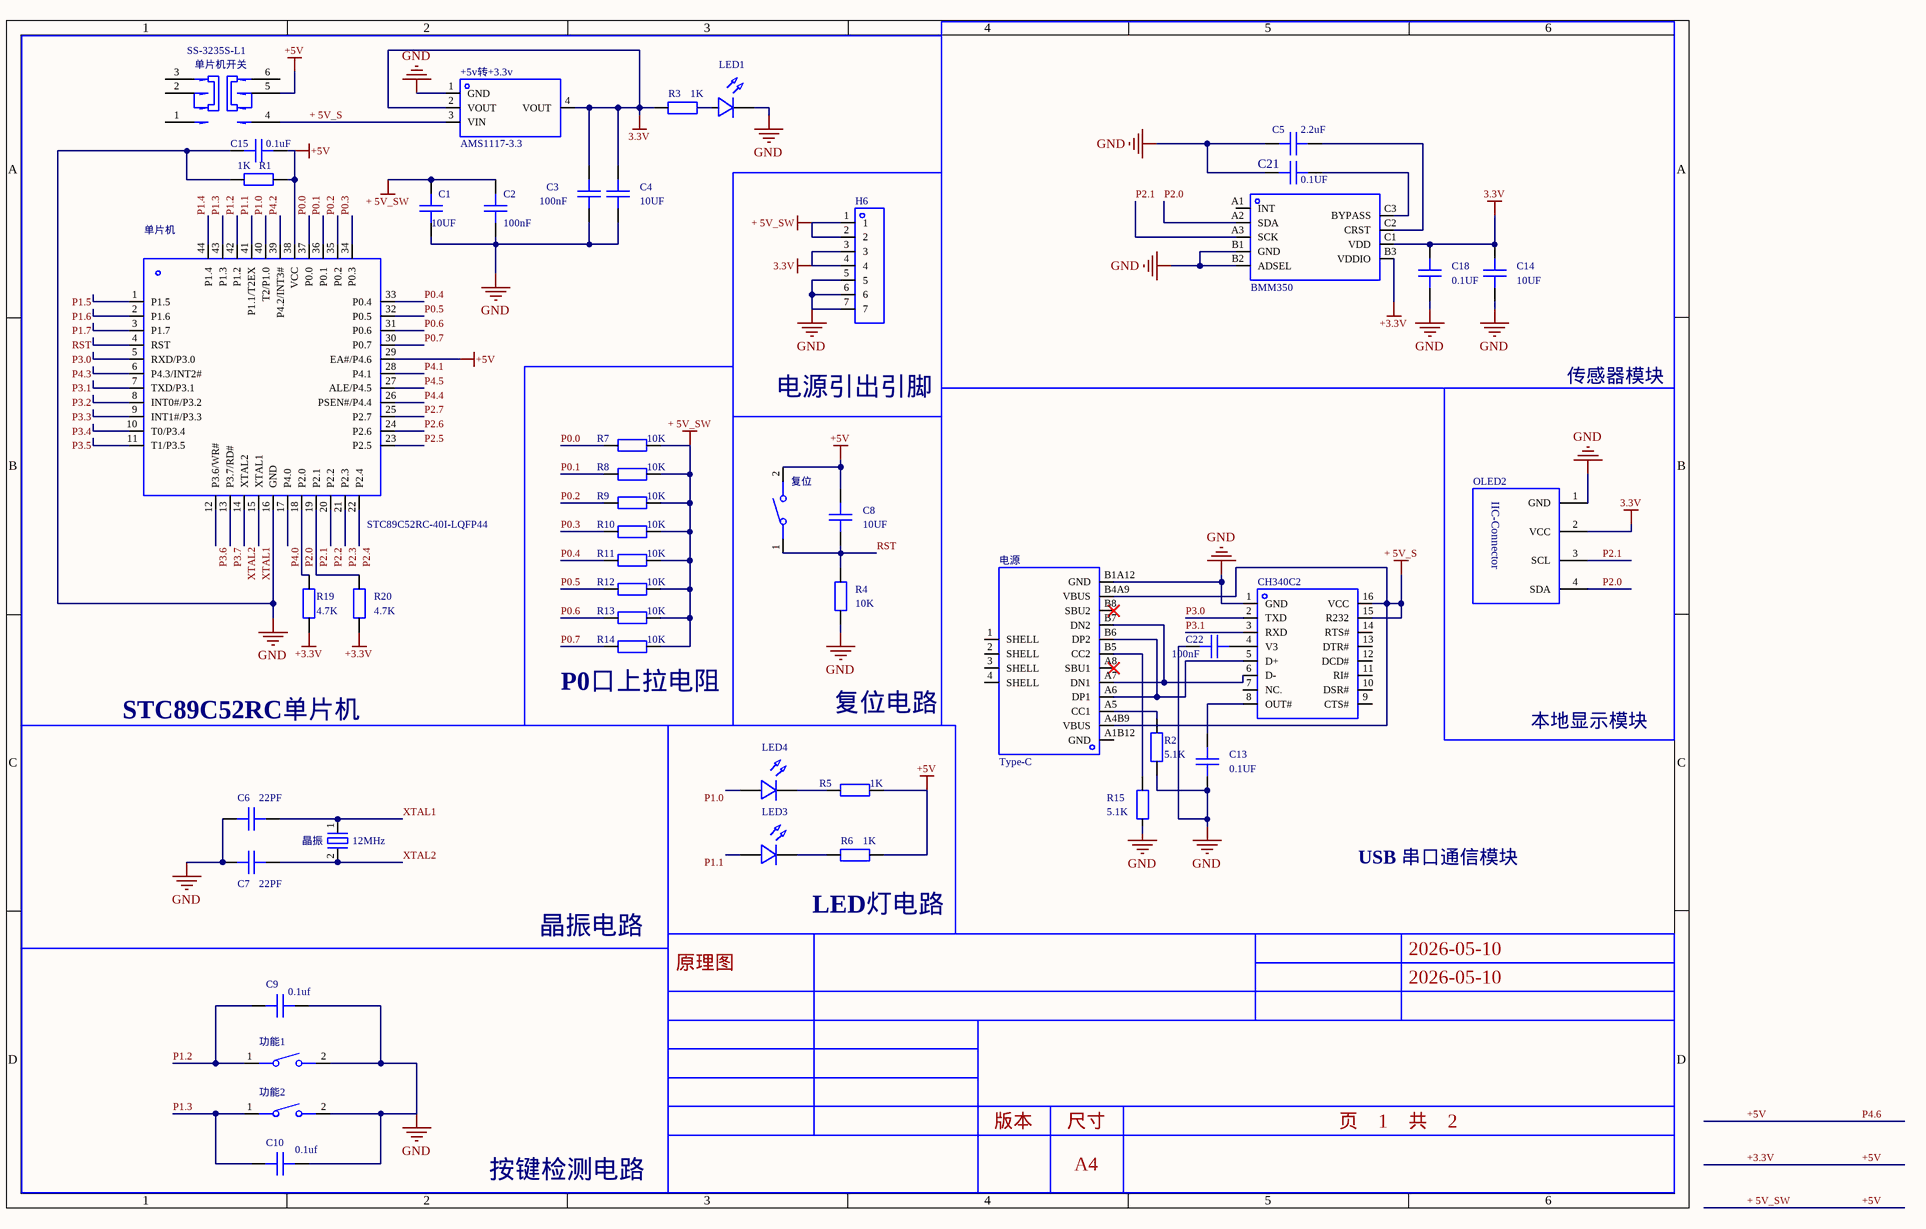
[diagram p0: MISC51448-3.schdoc]
# Altium project MISC51448-2.PrjPcb
1 sheet, 48 parts. Net scope: global (net labels, ports and power ports of the same name join across sheets).
Board file: MISC51448.pcbdoc

## Sheet MISC51448-3.schdoc
size 297 x 209 mm; Version: V1.0; @Project Name: MISC51448; @Page Count: 2; @Update Date: 2026-05-18; @Create Date: 2026-05-18; @Schematic Name: MISC51448; @Page No: 1; @Board Name: MISC51448; @Create Time: 00:24:12; @Update Time: 02:37:15; Size: A4

### Parts
+5v转+3.3v  AMS1117-3.3  [SOT-223-3_L6.5-W3.4-P2.30-LS7.0-BR]
C1  10UF  [C0805]
C2  100nF  [C0805]
C3  100nF  [C0805]
C4  10UF  [C0805]
C5  2.2uF  [C0805]
C6  22PF  [C0805]
C7  22PF  [C0805]
C8  10UF  [C0805]
C9  0.1uf  [C0805]
C10  0.1uf  [C0805]
C13  0.1UF  [C0805]
C14  10UF  [C0805]
C15  0.1uF  [C0805]
C18  0.1UF  [C0805]
C21  0.1UF  [C0805]
C22  100nF  [C0603]
CH340C2  CH340C  [SOP-16_L10.0-W3.9-P1.27-LS6.0-BL]  (value not drawn)
H6  (no value)  [HDR-TH_7P-P2.54-V-M]
LED1  (no value)  [LED_0805]
LED3  (no value)  [LED_0805]
LED4  (no value)  [LED_0805]
OLED2  0.96OLED_4P_MODULE_JX  [0.96OLED_4P]  (value not drawn)
R1  1K  [R0805]
R2  5.1K  [R0603]
R3  1K  [R0805]
R4  10K  [R0805]
R5  1K  [R0805]
R6  1K  [R0805]
R7  10K  [R0805]
R8  10K  [R0805]
R9  10K  [R0805]
R10  10K  [R0805]
R11  10K  [R0805]
R12  10K  [R0805]
R13  10K  [R0805]
R14  10K  [R0805]
R15  5.1K  [R0603]
R19  4.7K  [R0603]
R20  4.7K  [R0603]
U1  BMM350  [WLCSP-9_L1.3-W1.3-R3-C3-P0.40-TL]
功能1  轻触按键3*4*H  [SW-SMD_L4.0-W2.9-LS5.0]  (value not drawn)
功能2  轻触按键3*4*H  [SW-SMD_L4.0-W2.9-LS5.0]  (value not drawn)
单片机  STC89C52RC-40I-LQFP44  [LQFP-44_L10.0-W10.0-P0.80-LS12.0-BL]
单片机开关  SS-3235S-L1  [SW-SMD_SS-3235S-LX]
复位  轻触按键3*4*H  [SW-SMD_L4.0-W2.9-LS5.0]  (value not drawn)
晶振  12MHz  [CRYSTAL-SMD_L11.4-W4.7-LS12.7]
电源  Type-C  [USB-C-SMD_TYPE-C16PIN]

### Blocks framed on the sheet
传感器模块: C5 C14 C18 C21 U1
STC89C52RC单片机: +5v转+3.3v C1-C4 C15 LED1 R1 R3 R19 R20 单片机 单片机开关
电源引出引脚: H6
P0口上拉电阻: R7-R14
复位电路: C8 R4 复位

### Nets
3.3V: +5v转+3.3v.2(VOUT) +5v转+3.3v.4(VOUT) C3.2 C4.2 C14.1 C18.2 H6.3 H6.4 OLED2.2(VCC) R3.1 U1.C1(VDD)
+ 5V_S: +5v转+3.3v.3(VIN) CH340C2.15(R232) CH340C2.16(VCC) 单片机开关.4 电源.A4B9(VBUS) 电源.B4A9(VBUS)
+ 5V_SW: C1.2 C2.2 C8.1 C15.2 H6.1 H6.2 R1.2 R5.2 R6.2 R7.2 R8.2 R9.2 R10.2 R11.2 R12.2 R13.2 R14.2 R19.1 R20.1 U1.B3(VDDIO) 单片机.29(EA#/P4.6) 单片机.38(VCC) 单片机开关.5 复位.2  [also labelled +3.3V, +5V, P4.6]
GND: +5v转+3.3v.1(GND) C1.1 C2.1 C3.1 C4.1 C5.2 C6.2 C7.2 C9.1 C10.1 C13.1 C14.2 C15.1 C18.1 C21.1 C22.1 CH340C2.1(GND) H6.5 H6.6 H6.7 LED1.1(C) OLED2.1(GND) R1.1 R2.1 R4.1 R15.1 U1.B1(GND) U1.B2(ADSEL) 功能1.2 功能2.2 单片机.16(GND) 电源.B1A12(GND)
P0.0: R7.1 单片机.37(P0.0)
P0.1: R8.1 单片机.36(P0.1)
P0.2: R9.1 单片机.35(P0.2)
P0.3: R10.1 单片机.34(P0.3)
P0.4: R11.1 单片机.33(P0.4)
P0.5: R12.1 单片机.32(P0.5)
P0.6: R13.1 单片机.31(P0.6)
P0.7: R14.1 单片机.30(P0.7)
P1.0: LED4.2(A) 单片机.40(T2/P1.0)
P1.1: LED3.2(A) 单片机.41(P1.1/T2EX)
P1.2: C9.2 功能1.1 单片机.42(P1.2)
P1.3: C10.2 功能2.1 单片机.43(P1.3)
P1.4: 单片机.44(P1.4)
P1.5: 单片机.1(P1.5)
P1.6: 单片机.2(P1.6)
P1.7: 单片机.3(P1.7)
P2.0: OLED2.4(SDA) R19.2 U1.A2(SDA) 单片机.18(P2.0)
P2.1: OLED2.3(SCL) R20.2 U1.A3(SCK) 单片机.19(P2.1)
P2.2: 单片机.20(P2.2)
P2.3: 单片机.21(P2.3)
P2.4: 单片机.22(P2.4)
P2.5: 单片机.23(P2.5)
P2.6: 单片机.24(P2.6)
P2.7: 单片机.25(P2.7)
P3.0: CH340C2.2(TXD) 单片机.5(RXD/P3.0)
P3.1: CH340C2.3(RXD) 单片机.7(TXD/P3.1)
P3.2: 单片机.8(INT0#/P3.2)
P3.3: 单片机.9(INT1#/P3.3)
P3.4: 单片机.10(T0/P3.4)
P3.5: 单片机.11(T1/P3.5)
P3.6: 单片机.12(P3.6/WR#)
P3.7: 单片机.13(P3.7/RD#)
P4.0: 单片机.17(P4.0)
P4.1: 单片机.28(P4.1)
P4.2: 单片机.39(P4.2/INT3#)
P4.3: 单片机.6(P4.3/INT2#)
P4.4: 单片机.26(PSEN#/P4.4)
P4.5: 单片机.27(ALE/P4.5)
RST: C8.2 R4.2 单片机.4(RST) 复位.1
XTAL1: C6.1 单片机.15(XTAL1) 晶振.1
XTAL2: C7.1 单片机.14(XTAL2) 晶振.2(GND)
NetC5_1: C5.1 U1.C2(CRST)
NetC13_2: C13.2 CH340C2.8(OUT#)
NetC21_2: C21.2 U1.C3(BYPASS)
NetC22_2: C22.2 CH340C2.4(V3)
NetCH340C2_5: CH340C2.5(D+) 电源.A6(DP1) 电源.B6(DP2)
NetCH340C2_6: CH340C2.6(D-) 电源.A7(DN1) 电源.B7(DN2)
NetLED1_2: LED1.2(A) R3.2
NetLED3_1: LED3.1(C) R6.1
NetLED4_1: LED4.1(C) R5.1
NetR2_2: R2.2 电源.A5(CC1)
NetR15_2: R15.2 电源.B5(CC2)

Not connected (* = marked no-connect by the designer): CH340C2 7(NC.) 9(CTS#) 10(DSR#) 11(RI#) 12(DCD#) 13(DTR#) 14(RTS#); U1 A1(INT); 单片机开关 1 2 3 6; 电源 1(SHELL) 2(SHELL) 3(SHELL) 4(SHELL) A1B12(GND) A8(SBU1)* B8(SBU2)*

### Notes on the sheet
- 本地显示模块
- USB 串口通信模块
- 晶振电路
- LED灯电路
- 按键检测电路
- 2026-05-10
- 原理图
- 版本
- 尺寸
- A4
- 页    1    共    2

### Library data of the parts
+5v转+3.3v = AMS1117-3.3_C6186: 输出类型:固定;工作电压:15V;输出电压:3.3V;输出电流:1A;电源纹波抑制比(PSRR):72dB@(120Hz);输出极性:正极;; Manufacturer: AMS; AddInBom: yes; Output Type: 固定; Voltage - Supply: 15V; Output Voltage: 3.3V; Output Current: 1A; Voltage Dropout: 1.1V@(800mA); standby current: 5mA; Noise: 0.003%Vout; Output Configuration: 正极; Number of Outputs: 1; ModelId: 925194bf9823436183a3e0b978a8d076; ModelName: SOT-223-4P_L6.5-W3.5-H1.6-LS7.0-P2.30; ModelTransform: 279.89794,255.905,0,180,0,0,-3.9385,-0.0005,0; Device: AMS1117-3.3_C6186; Symbol: AMS1117-3.3; FootprintName: SOT-223-3_L6.5-W3.4-P2.30-LS7.0-BR; LCSC Part Name: 3.3V 1A 15V; SupplierPart: C6186; ManufacturerPart: AMS1117-3.3; Supplier Footprint: SOT-223; JLCPCB Part Class: 基础库; Datasheet: https://item.szlcsc.com/datasheet/AMS1117-3.3/6652.html; Supplier: LCSC; ConvertToPcb: yes; Power Supply Rejection Ratio (PSRR): 72dB@(120Hz); Features: 过流保护；热关断; Operating Temperature: -40℃~+125℃
C1-C4 C8 = CAP_0805: Symbol: Capacitance; ConvertToPcb: yes; ModelId: 1ba041120af144c991958decab20d241; ModelName: C0805_L2.0-W1.3-H1.3; ModelTransform: 78.74,51.181,0,0,0,0,0,0.0005,0; Device: CAP_0805; FootprintName: C0805; AddInBom: yes; Supplier Footprint: 0805
  C1 C4 C8: Value: 10UF
  C2 C3: Value: 100nF
C5 = CGB4B3X7R0J225K055AB: 容值:2.2uF;精度:±10%;额定电压:6.3V;材质(温度系数):X7R;; Manufacturer: TDK; 3D Model: 1ba041120af144c991958decab20d2410819f05c4eef4c71ace90d822a990e87; 3D Model Transform: 78.74,51.181,0,0,0,0,0,0.0005,0; Tolerance: ±10%; Voltage Rated: 6.3V; Temperature Coefficient: X7R; AddInBom: yes; ModelName: C0805_L2.0-W1.3-H1.3; Device: CGB4B3X7R0J225K055AB; Symbol: CGB4B3X7R0J225K055AB; LCSC Part Name: 2.2uF ±10% 6.3V; Supplier Part: C2179322; Manufacturer Part: CGB4B3X7R0J225K055AB; Supplier Footprint: 0805; JLCPCB Part Class: Extended Part; Datasheet: https://atta.szlcsc.com/upload/public/pdf/source/20191105/C343012_3F47E91403558E3EBEE82CA44A798D40.pdf; Supplier: LCSC; Value: 2.2uF; FootprintName: C0805; ConvertToPcb: yes
C6 C7 C9 C10 = CAP_0805: SymbolName: Capacitance; ConvertToPcb: yes; ModelId: 1ba041120af144c991958decab20d241; ModelName: C0805_L2.0-W1.3-H1.3; ModelTransform: 78.74,51.181,0,0,0,0,0,0.0005,0; Device: CAP_0805; FootprintName: C0805; AddInBom: yes; Supplier Footprint: 0805
  C6 C7: Value: 22PF
  C9 C10: Value: 0.1uf
C13-C15 C18 C21 = CAP_0805: Symbol: Capacitance; 3D Model: 1ba041120af144c991958decab20d241; 3D Model Transform: 78.74,51.181,0,0,0,0,0,0.0005,0; ConvertToPcb: yes; ModelName: C0805_L2.0-W1.3-H1.3; Device: CAP_0805; Supplier Footprint: 0805; FootprintName: C0805; AddInBom: yes
  C13 C18 C21: Value: 0.1UF
  C14: Value: 10UF
  C15: Value: 0.1uF
C22 = CAP_0603: Symbol: Capacitance; 3D Model: ac125912035d415993ca9572d50418b1; 3D Model Transform: 62.992,31.496,0,0,0,0,0,0,0; ConvertToPcb: yes; ModelName: C0603_L1.6-W0.8-H0.8; Device: CAP_0603; Supplier Footprint: 0603; Value: 100nF; FootprintName: C0603; AddInBom: yes
CH340C2 = CH340C: 应用功能:收发器;USB协议版本:USB 2.0;数据速率:2Mbps;; Manufacturer: WCH(南京沁恒); 3D Model: 3361a6792abf4a8f8fbca4f1924a67ee; 3D Model Transform: 240.39054,393.7,0,90,0,0,0,0,0; Applications Function: 收发器; USB Protocol: USB 2.0; Voltage - Supply: 3.3V；5V; Data Rate: 2Mbps; Current - Supply: 7mA; Supply Current (Iq): 50uA; AddInBom: yes; ModelName: SOP-16_L9.9-W3.9-H1.5-LS6.0-P1.27; Device: CH340C; Symbol: CH340C; LCSC Part Name: USB转串口芯片; Supplier Part: C84681; Manufacturer Part: CH340C; Supplier Footprint: SOP-16; JLCPCB Part Class: 扩展库; Datasheet: https://item.szlcsc.com/datasheet/CH340C/85852.html; Supplier: LCSC; Operating Temperature: -20℃~+70℃; FootprintName: SOP-16_L10.0-W3.9-P1.27-LS6.0-BL; ConvertToPcb: yes
H6 = HDR-M_2.54_1x7P: Symbol: PZ254V-11-07P; ConvertToPcb: yes; ModelId: 3f496cdc752348c6a5e9157bbaceaf96; ModelName: HDR-TH_7P-P2.54-M-LI-1X7P; ModelTransform: 690.1561,98.425,0,0,0,0,0,0,-118.11; Device: HDR-M_2.54_1x7P; FootprintName: HDR-TH_7P-P2.54-V-M; AddInBom: yes; SupplierPart: C492406; Supplier Footprint: 插件
LED1 LED3 LED4 = LED_0805-G: Symbol: LED_G; Convert to PCB: yes; 3D Model: 381ae4d721d6485eaad9d0ca067812b5; 3D Model Transform: 63.9,39.8,31.9,0,0,0,0,0,0; ModelName: LED-0805_G; Device: LED_0805-G; Add into BOM: yes; Supplier Footprint: 0805; FootprintName: LED_0805
OLED2 = 0.96OLED_4P_MODULE_JX: 3D Model: 79c000fdb68d45a296c2e9bedf4f9055; 3D Model Transform: 1393.69792,1318.895,0,0,0,0,0,-560.079,-137.795; AddInBom: yes; Device: 0.96OLED_4P_MODULE_JX; Symbol: 0.96OLED_4P_MODULE_JX; LCSC Part Name: 0.96OLED_4P_MODULE_JX; Supplier Part: C9900004566; Manufacturer Part: 0.96OLED_4P_MODULE_JX; Supplier Footprint: 插件; JLCPCB Part Class: 扩展库; Supplier: LCSC; FootprintName: 0.96OLED_4P; ConvertToPcb: yes; ModelName: 0.96OLED_4P
R1 = Res_0805: Symbol: 电阻; 3D Model: 37a81e68749a4138bd2dfa6897b24b85; 3D Model Transform: 78.74,51.181,0,0,0,0,0,-0.0005,0; ConvertToPcb: yes; ModelName: R0805_L2.0-W1.3-H0.6; Device: Res_0805; Supplier Footprint: 0805; Value: 1K; FootprintName: R0805; AddInBom: yes
R2 R15 = Res_0603: Symbol: 电阻; 3D Model: fc143cca1e79419f9cd78b61e9279f08; 3D Model Transform: 31.8897,63.7794,0,90,0,0,0,0,0; ConvertToPcb: yes; Device: Res_0603; Value: 5.1K; Supplier Footprint: 0603; FootprintName: R0603; AddInBom: yes; ModelName: R0603
R3 R4 R7-R14 = Res_0805: Symbol: 电阻; ConvertToPcb: yes; ModelId: 349bb002ce6c6897; ModelName: R0805_L2.0-W1.3-H0.6; ModelTransform: 0,0,0,0,0,0,0,0,0; Device: Res_0805; FootprintName: R0805; AddInBom: yes; Supplier Footprint: 0805
  R3: Value: 1K
  R4 R7-R14: Value: 10K
R5 R6 = Res_0805: SymbolName: 电阻; ConvertToPcb: yes; ModelId: 349bb002ce6c6897; ModelName: R0805_L2.0-W1.3-H0.6; ModelTransform: 0,0,0,0,0,0,0,0,0; Device: Res_0805; Value: 1K; FootprintName: R0805; AddInBom: yes; Supplier Footprint: 0805
R19 R20 = Res_0603: Symbol: 电阻; ConvertToPcb: yes; ModelId: c5da5eb17d71f24d; ModelTransform: 0,0,0,0,0,0,0,0,0; Device: Res_0603; Value: 4.7K; FootprintName: R0603; AddInBom: yes; Supplier Footprint: 0603; ModelName: R0603
U1 = BMM350: 3D Model: 5e906eb31187499fa9dbe78db1290694; 3D Model Transform: 51.5747,51.181,0,0,0,0,0,0,0; AddInBom: yes; Device: BMM350; Symbol: BMM350; LCSC Part Name: BMM350; Supplier Part: C7496950; Manufacturer Part: BMM350; Supplier Footprint: BGA-9_1.28X1.28mm; JLCPCB Part Class: 扩展库; Supplier: LCSC; FootprintName: WLCSP-9_L1.3-W1.3-R3-C3-P0.40-TL; ConvertToPcb: yes; ModelName: WLCSP-9_L1.3-W1.3-R3-C3-P0.40-TL
功能1 功能2 复位 = 轻触按键3*4*H: AddInBom: yes; ModelId: 63599cce708d48afbce1b0db00354477; ModelName: SW-SMD_L4.0-W2.9-H2-LS5.0; ModelTransform: 196.85,114.173,0,0,0,0,0,0,0; Device: 轻触按键3*4*H; Symbol: 轻触按键3*4*H; FootprintName: SW-SMD_L4.0-W2.9-LS5.0; LCSC Part Name: 轻触按键3*4*H; SupplierPart: C9900017573; ManufacturerPart: 轻触按键3*4*H; Supplier Footprint: 轻触按键3*4*2.5; JLCPCB Part Class: 扩展库; Supplier: LCSC; ConvertToPcb: yes
单片机 = STC89C52RC-40I-LQFP44: CPU内核:51家族;; Manufacturer: STC; Symbol: STC89C52RC-40I_C8707; AddInBom: yes; CPU Core: 51家族; Program Storage Size: 8KB; Program Memory Type: FLASH; Number of I/O: 39; Voltage - Supply: 3.3V~5.5V; ModelId: cfc67ede9fd147078f17820e55193bca; ModelName: LQFP-44_L10.0-W10.0-H1.4-LS12.0-P0.80; ModelTransform: 472.441,472.441,0,0,0,0,0,0,0; Device: STC89C52RC-40I-LQFP44; FootprintName: LQFP-44_L10.0-W10.0-P0.80-LS12.0-BL; LCSC Part Name: 单片机原理及应用; SupplierPart: C8707; ManufacturerPart: STC89C52RC-40I-LQFP44; Supplier Footprint: LQFP-44(10x10); JLCPCB Part Class: 扩展库; Datasheet: https://item.szlcsc.com/datasheet/STC89C52RC-40I-LQFP44/9213.html; Supplier: LCSC; ConvertToPcb: yes
单片机开关 = SS-3235S-L1: 电路结构:双刀双掷;安装方式:卧贴;开关颜色:黑色;额定电流:50mA;额定电压:12V;工作寿命:1万次;; Manufacturer: XKB Connection(中国星坤); AddInBom: yes; Circuit: 双刀双掷; Actuator Style: 矩形柱状; Switch Height: 3.2mm; Actuator Color: 黑色; Current Rating: 50mA; Voltage Rating: 12V; Life: 1万次; ModelId: 81e407adedd8b3e1; ModelTransform: 0,0,0,0,0,0,0,0,0; Device: SS-3235S-L1; Symbol: SS-3235S-L1; FootprintName: SW-SMD_SS-3235S-LX; LCSC Part Name: 柄长2mm 卧贴双档 滑动开关; SupplierPart: C500055; ManufacturerPart: SS-3235S-L1; Supplier Footprint: SMD,9.1x3.6mm; JLCPCB Part Class: 扩展库; Datasheet: https://item.szlcsc.com/datasheet/SS-3235S-L1/512181.html; Supplier: LCSC; ConvertToPcb: yes; Termination Style: 鸥翼型; Length: 9.1mm; Width: 3.55mm; Mounting Type: 卧贴; Operating Temperature: -40℃~+85℃; ModelName: SW-SMD_SS-3235S-LX
晶振 = ABLS-12.000MHZ-B4H-T: 频率:12MHz;常温频差:±30ppm;负载电容:18pF;频率稳定度:±35ppm;; Manufacturer: ABRACON; AddInBom: yes; Normal temperature Frequency Tolerance: ±30ppm; Load Capacitance: 18pF; Frequency Stability: ±35ppm; Equivalent Series Resistance(ESR): 50Ω; ModelId: be19d32e6d024fb4863eb8f4e3f5efcc; ModelTransform: 499.999,185.039,0,0,0,0,0,0,0; Device: ABLS-12.000MHZ-B4H-T; Symbol: ABLS-12.000MHZ-B4H-T; FootprintName: CRYSTAL-SMD_L11.4-W4.7-LS12.7; LCSC Part Name: 12MHz ±30ppm 18pF; SupplierPart: C1986452; ManufacturerPart: ABLS-12.000MHZ-B4H-T; Supplier Footprint: HC-49S-SMD; JLCPCB Part Class: 扩展库; Datasheet: https://item.szlcsc.com/datasheet/ABLS-12.000MHZ-B4H-T/2077997.html; Supplier: LCSC; ConvertToPcb: yes; Value: 12MHz; Operating Temperature: -20℃~+70℃; ModelName: CRYSTAL-SMD_L11.4-W4.7-LS12.7
电源 = Type-C-TOP_1: 3D Model: d6783d3a2268456b863f42d3286191d0; 3D Model Transform: 351.9678,311.023,0,180,0,0,0,-41.85,-39.37; AddInBom: yes; Device: Type-C-TOP_1; Symbol: TYPE-C-TOP_1; LCSC Part Name: Type-C-TOP_1; Supplier Part: C9900005857; Manufacturer Part: Type-C; Supplier Footprint: Type-C16P; JLCPCB Part Class: 扩展库; Supplier: LCSC; FootprintName: USB-C-SMD_TYPE-C16PIN; ConvertToPcb: yes; ModelName: USB-C-SMD_TYPE-C16PIN